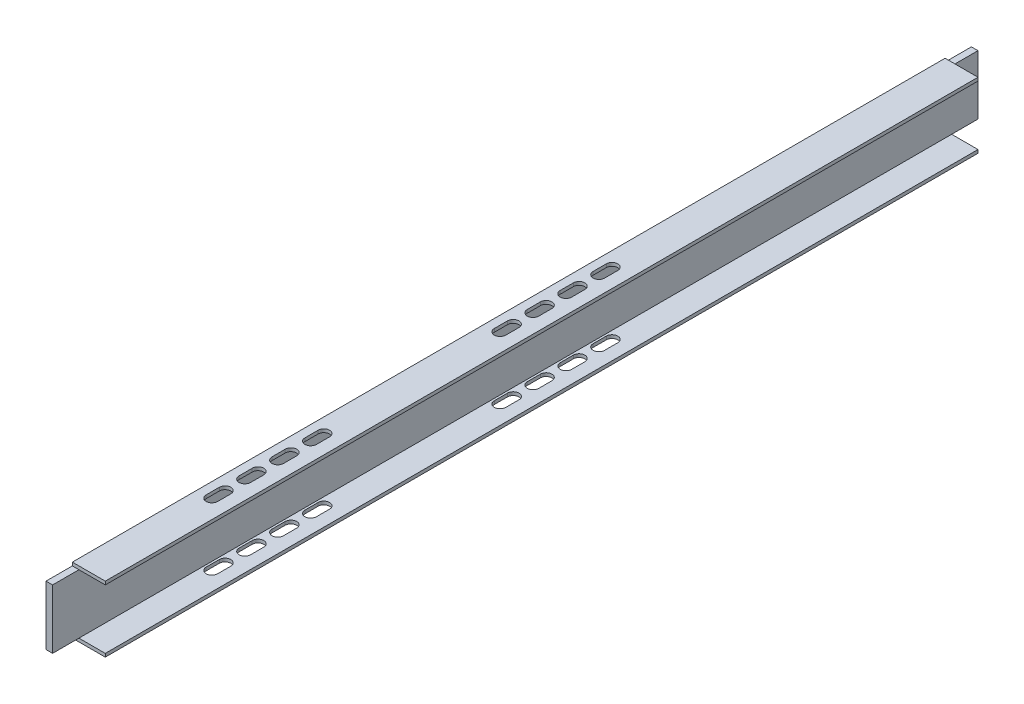
SolidWorks part; units mm, degrees
ref_plane "Front Plane" through (0, 0, 0) normal (0, 0, 1) x (1, 0, 0)
ref_plane "Top Plane" through (0, 0, 0) normal (0, 1, 0) x (1, 0, 0)
ref_plane "Right Plane" through (0, 0, 0) normal (1, 0, 0) x (0, 0, -1)
sketch "Sketch1" plane through (0, 0, 0) normal (0, 0, 1) x (1, 0, 0)
  line L0 (0, 0) -> (-40, 0)
  line L1 (-40, 0) -> (-40, 80)
  line L2 (-40, 80) -> (0, 80)
  line L3 (0, 80) -> (0, 76)
  line L4 (0, 76) -> (-32, 76)
  line L5 (-32, 76) -> (-32, 4)
  line L6 (-32, 4) -> (0, 4)
  line L7 (0, 4) -> (0, 0)
  dimension "D1" = 80
  dimension "D2" = 40
  dimension "D3" = 40
  dimension "D4" = 4
  dimension "D5" = 4
  dimension "D6" = 8
sheet metal parameters "Sheet metal 1" thickness 3 parameters "D1"=3
extrude "Extrude1" add sketch "Sketch1" along normal blind 1124
sketch "Sketch2" plane through (0, 80, 0) normal (0, 1, 0) x (1, 0, 0)
  line L0 (-40, -1124) -> (-40, 0) construction
  line L1 (0, 0) -> (-32, 0)
  line L2 (0, 0) -> (0, -32)
  line L3 (0, -32) -> (-32, -32)
  line L4 (-32, 0) -> (-32, -32)
  line L6 (0, -1124) -> (-32, -1124)
  line L7 (0, -1124) -> (0, -1092)
  line L8 (0, -1092) -> (-32, -1092)
  line L9 (-32, -1124) -> (-32, -1092)
  dimension "D1" = 8
  dimension "D2" = 32
  dimension "D3" = 8
  dimension "D4" = 32
extrude "Cut-Extrude1" cut sketch "Sketch2" against normal through all
sketch "Sketch3" plane through (-32, 0, 0) normal (1, 0, 0) x (0, 0, -1)
  line L1 (-1092, 76) -> (-1124, 76)
  line L2 (-1092, 76) -> (-1092, 80)
  line L3 (-1092, 80) -> (-1124, 80)
  line L4 (-1124, 76) -> (-1124, 80)
  line L5 (-1092, 4) -> (-1124, 4)
  line L6 (-1092, 4) -> (-1092, 0)
  line L7 (-1092, 0) -> (-1124, 0)
  line L8 (-1124, 4) -> (-1124, 0)
  line L9 (-32, 76) -> (0, 76)
  line L10 (-32, 76) -> (-32, 80)
  line L11 (-32, 80) -> (0, 80)
  line L12 (0, 76) -> (0, 80)
  line L14 (-32, 4) -> (0, 4)
  line L15 (-32, 4) -> (-32, 0)
  line L16 (-32, 0) -> (0, 0)
  line L17 (0, 4) -> (0, 0)
extrude "Cut-Extrude2" cut sketch "Sketch3" against normal blind 1200
sketch "Sketch4" plane through (0, 80, 0) normal (0, 1, 0) x (1, 0, 0)
  line L0 (-22.5, -924) -> (-22.5, -940) construction
  line L1 (0, -1092) -> (0, -32) construction
  line L2 (-29.5, -924) -> (-29.5, -940)
  line L3 (-15.5, -924) -> (-15.5, -940)
  arc A0 (-29.5, -924) -> (-15.5, -924) centre (-22.5, -924) cw
  arc A1 (-29.5, -940) -> (-15.5, -940) centre (-22.5, -940) ccw
  point P5 (-22.5, -932)
  dimension "D1" = 22.5
  dimension "D2" = 160
  dimension "D3" = 16
  dimension "D4" = 7
  dimension "D5" = 7
extrude "Cut-Extrude3" cut sketch "Sketch4" against normal through all
pattern_linear "LPattern1" count 4 spacing 40 along (0, 0, -1) of "Cut-Extrude3"
pattern_linear "LPattern2" count 2 spacing 350 along (0, 0, -1) of "Cut-Extrude3", "LPattern1"
